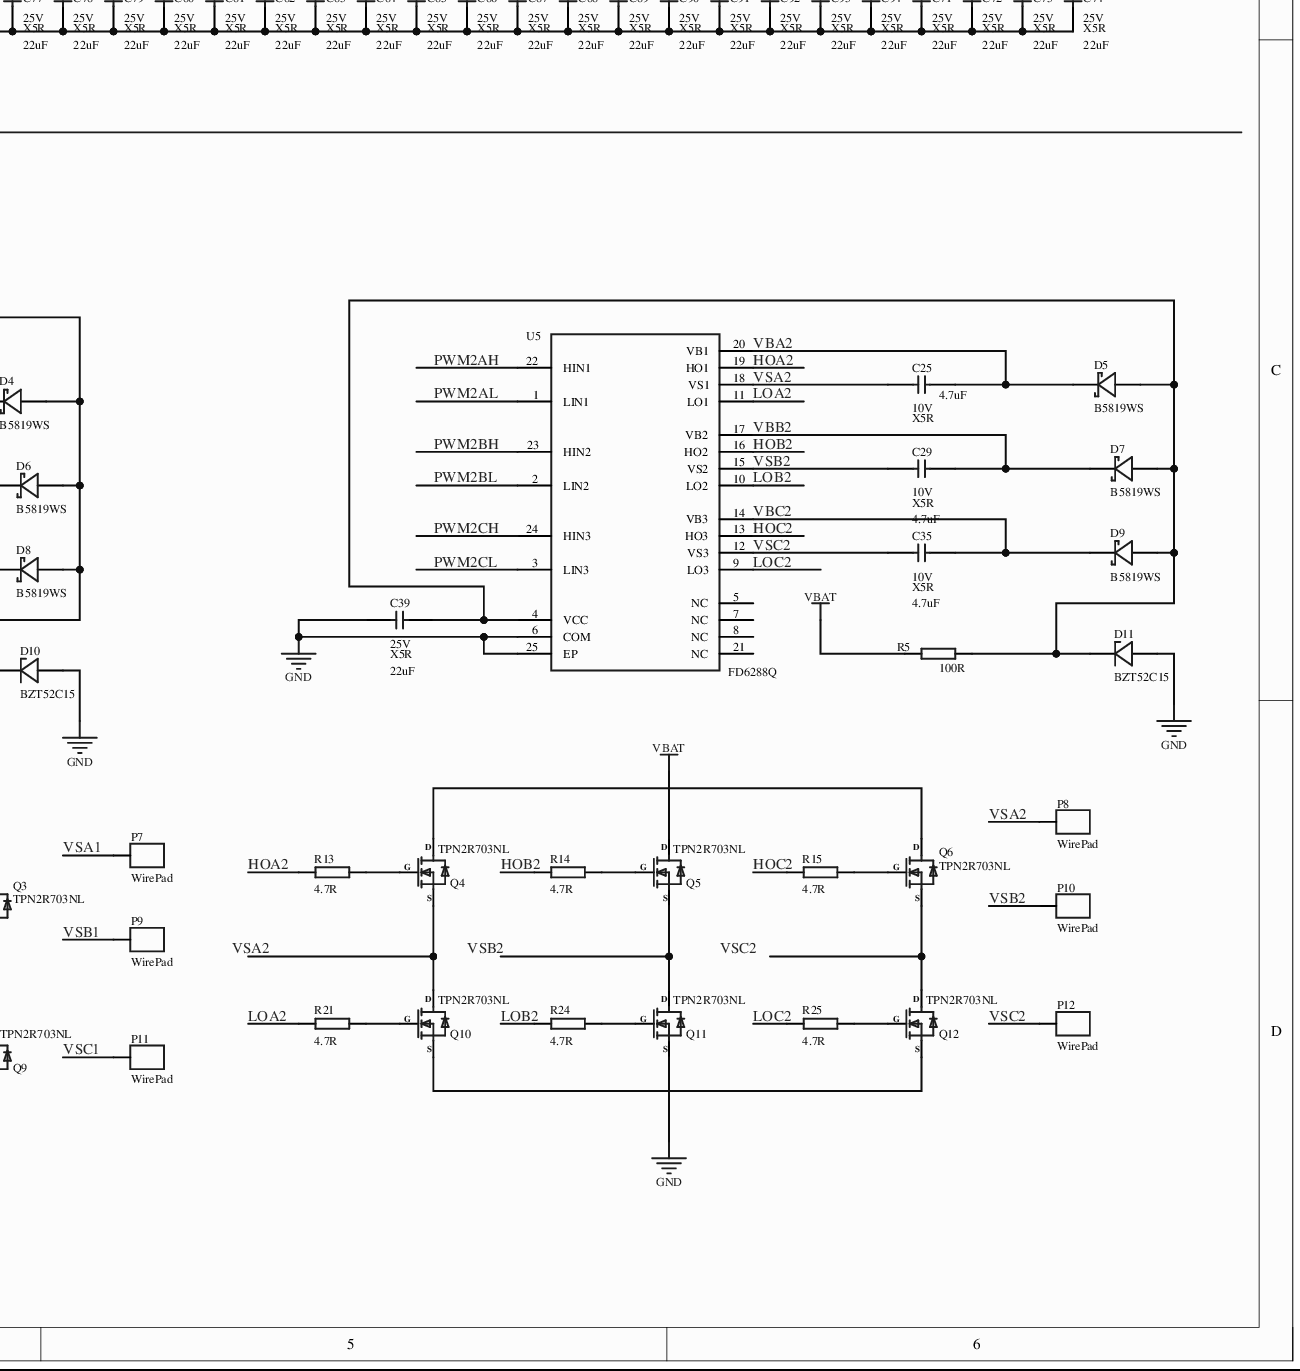
[diagram p0: MISC49862-3.schdoc, bottom right]
# Altium project MISC49862-2.PrjPcb (part 3 of 4)
## Sheet MISC49862-3.schdoc (continued)
### Library data of the parts (continued)
C71 = =Value +' '+ Voltage + ' ' + Type: SMD ceramic capacitor; MLCC; 0805(2012);; Device: 22uF 25V X5R; Symbol: 22uF 0805 25V X5R; Origin Footprint 2: CAPC2012[0805]; Origin Footprint 3: CAPC2012[0805]S-L; Origin Footprint 4: CAPC2012[0805]S-M; UniqueId: 13c458815c86755b; AddInBom: yes; Origin Footprint 1: CAPC2012[0805]S-N; Design Item ID: 22uF 0805 25V X5R; Library Name: SEEKFREE_Capacitor; Revision: V1.0; FootprintName: CAPC2012[0805]S-N; ConvertToPcb: yes
C72 = =Value +' '+ Voltage + ' ' + Type: SMD ceramic capacitor; MLCC; 0805(2012);; Device: 22uF 25V X5R; Symbol: 22uF 0805 25V X5R; Origin Footprint 2: CAPC2012[0805]; Origin Footprint 3: CAPC2012[0805]S-L; Origin Footprint 4: CAPC2012[0805]S-M; UniqueId: 4c445f6b18a98c19; AddInBom: yes; Origin Footprint 1: CAPC2012[0805]S-N; Design Item ID: 22uF 0805 25V X5R; Library Name: SEEKFREE_Capacitor; Revision: V1.0; FootprintName: CAPC2012[0805]S-N; ConvertToPcb: yes
C73 = =Value +' '+ Voltage + ' ' + Type: SMD ceramic capacitor; MLCC; 0805(2012);; Device: 22uF 25V X5R; Symbol: 22uF 0805 25V X5R; Origin Footprint 2: CAPC2012[0805]; Origin Footprint 3: CAPC2012[0805]S-L; Origin Footprint 4: CAPC2012[0805]S-M; UniqueId: ed67743022cf1596; AddInBom: yes; Origin Footprint 1: CAPC2012[0805]S-N; Design Item ID: 22uF 0805 25V X5R; Library Name: SEEKFREE_Capacitor; Revision: V1.0; FootprintName: CAPC2012[0805]S-N; ConvertToPcb: yes
C74 = =Value +' '+ Voltage + ' ' + Type: SMD ceramic capacitor; MLCC; 0805(2012);; Device: 22uF 25V X5R; Symbol: 22uF 0805 25V X5R; Origin Footprint 2: CAPC2012[0805]; Origin Footprint 3: CAPC2012[0805]S-L; Origin Footprint 4: CAPC2012[0805]S-M; UniqueId: 428606a84a8f4e02; AddInBom: yes; Origin Footprint 1: CAPC2012[0805]S-N; Design Item ID: 22uF 0805 25V X5R; Library Name: SEEKFREE_Capacitor; Revision: V1.0; FootprintName: CAPC2012[0805]S-N; ConvertToPcb: yes
C75 = =Value +' '+ Voltage + ' ' + Type: SMD ceramic capacitor; MLCC; 0805(2012);; Device: 22uF 25V X5R; Symbol: 22uF 0805 25V X5R; Origin Footprint 2: CAPC2012[0805]; Origin Footprint 3: CAPC2012[0805]S-L; Origin Footprint 4: CAPC2012[0805]S-M; UniqueId: 94802851accbed84; AddInBom: yes; Origin Footprint 1: CAPC2012[0805]S-N; Design Item ID: 22uF 0805 25V X5R; Library Name: SEEKFREE_Capacitor; Revision: V1.0; FootprintName: CAPC2012[0805]S-N; ConvertToPcb: yes
C76 = =Value +' '+ Voltage + ' ' + Type: SMD ceramic capacitor; MLCC; 0805(2012);; Device: 22uF 25V X5R; Symbol: 22uF 0805 25V X5R; Origin Footprint 2: CAPC2012[0805]; Origin Footprint 3: CAPC2012[0805]S-L; Origin Footprint 4: CAPC2012[0805]S-M; UniqueId: e46c4319d3798579; AddInBom: yes; Origin Footprint 1: CAPC2012[0805]S-N; Design Item ID: 22uF 0805 25V X5R; Library Name: SEEKFREE_Capacitor; Revision: V1.0; FootprintName: CAPC2012[0805]S-N; ConvertToPcb: yes
C77 = =Value +' '+ Voltage + ' ' + Type: SMD ceramic capacitor; MLCC; 0805(2012);; Device: 22uF 25V X5R; Symbol: 22uF 0805 25V X5R; Origin Footprint 2: CAPC2012[0805]; Origin Footprint 3: CAPC2012[0805]S-L; Origin Footprint 4: CAPC2012[0805]S-M; UniqueId: d85eccf1df583bf1; AddInBom: yes; Origin Footprint 1: CAPC2012[0805]S-N; Design Item ID: 22uF 0805 25V X5R; Library Name: SEEKFREE_Capacitor; Revision: V1.0; FootprintName: CAPC2012[0805]S-N; ConvertToPcb: yes
C78 = =Value +' '+ Voltage + ' ' + Type: SMD ceramic capacitor; MLCC; 0805(2012);; Device: 22uF 25V X5R; Symbol: 22uF 0805 25V X5R; Origin Footprint 2: CAPC2012[0805]; Origin Footprint 3: CAPC2012[0805]S-L; Origin Footprint 4: CAPC2012[0805]S-M; UniqueId: 289a7498a46a83c5; AddInBom: yes; Origin Footprint 1: CAPC2012[0805]S-N; Design Item ID: 22uF 0805 25V X5R; Library Name: SEEKFREE_Capacitor; Revision: V1.0; FootprintName: CAPC2012[0805]S-N; ConvertToPcb: yes
C79 = =Value +' '+ Voltage + ' ' + Type: SMD ceramic capacitor; MLCC; 0805(2012);; Device: 22uF 25V X5R; Symbol: 22uF 0805 25V X5R; Origin Footprint 2: CAPC2012[0805]; Origin Footprint 3: CAPC2012[0805]S-L; Origin Footprint 4: CAPC2012[0805]S-M; UniqueId: 1d1687b72a359977; AddInBom: yes; Origin Footprint 1: CAPC2012[0805]S-N; Design Item ID: 22uF 0805 25V X5R; Library Name: SEEKFREE_Capacitor; Revision: V1.0; FootprintName: CAPC2012[0805]S-N; ConvertToPcb: yes
C80 = =Value +' '+ Voltage + ' ' + Type: SMD ceramic capacitor; MLCC; 0805(2012);; Device: 22uF 25V X5R; Symbol: 22uF 0805 25V X5R; Origin Footprint 2: CAPC2012[0805]; Origin Footprint 3: CAPC2012[0805]S-L; Origin Footprint 4: CAPC2012[0805]S-M; UniqueId: 2dbd9816442fdb9a; AddInBom: yes; Origin Footprint 1: CAPC2012[0805]S-N; Design Item ID: 22uF 0805 25V X5R; Library Name: SEEKFREE_Capacitor; Revision: V1.0; FootprintName: CAPC2012[0805]S-N; ConvertToPcb: yes
C81 = =Value +' '+ Voltage + ' ' + Type: SMD ceramic capacitor; MLCC; 0805(2012);; Device: 22uF 25V X5R; Symbol: 22uF 0805 25V X5R; Origin Footprint 2: CAPC2012[0805]; Origin Footprint 3: CAPC2012[0805]S-L; Origin Footprint 4: CAPC2012[0805]S-M; UniqueId: bdf2686215596067; AddInBom: yes; Origin Footprint 1: CAPC2012[0805]S-N; Design Item ID: 22uF 0805 25V X5R; Library Name: SEEKFREE_Capacitor; Revision: V1.0; FootprintName: CAPC2012[0805]S-N; ConvertToPcb: yes
C82 = =Value +' '+ Voltage + ' ' + Type: SMD ceramic capacitor; MLCC; 0805(2012);; Device: 22uF 25V X5R; Symbol: 22uF 0805 25V X5R; Origin Footprint 2: CAPC2012[0805]; Origin Footprint 3: CAPC2012[0805]S-L; Origin Footprint 4: CAPC2012[0805]S-M; UniqueId: 2ac4a713bdb27458; AddInBom: yes; Origin Footprint 1: CAPC2012[0805]S-N; Design Item ID: 22uF 0805 25V X5R; Library Name: SEEKFREE_Capacitor; Revision: V1.0; FootprintName: CAPC2012[0805]S-N; ConvertToPcb: yes
C83 = =Value +' '+ Voltage + ' ' + Type: SMD ceramic capacitor; MLCC; 0805(2012);; Device: 22uF 25V X5R; Symbol: 22uF 0805 25V X5R; Origin Footprint 2: CAPC2012[0805]; Origin Footprint 3: CAPC2012[0805]S-L; Origin Footprint 4: CAPC2012[0805]S-M; UniqueId: 2b2365c2d0e3ae99; AddInBom: yes; Origin Footprint 1: CAPC2012[0805]S-N; Design Item ID: 22uF 0805 25V X5R; Library Name: SEEKFREE_Capacitor; Revision: V1.0; FootprintName: CAPC2012[0805]S-N; ConvertToPcb: yes
C84 = =Value +' '+ Voltage + ' ' + Type: SMD ceramic capacitor; MLCC; 0805(2012);; Device: 22uF 25V X5R; Symbol: 22uF 0805 25V X5R; Origin Footprint 2: CAPC2012[0805]; Origin Footprint 3: CAPC2012[0805]S-L; Origin Footprint 4: CAPC2012[0805]S-M; UniqueId: ac7cf9eb5671d2c3; AddInBom: yes; Origin Footprint 1: CAPC2012[0805]S-N; Design Item ID: 22uF 0805 25V X5R; Library Name: SEEKFREE_Capacitor; Revision: V1.0; FootprintName: CAPC2012[0805]S-N; ConvertToPcb: yes
C85 = =Value +' '+ Voltage + ' ' + Type: SMD ceramic capacitor; MLCC; 0805(2012);; Device: 22uF 25V X5R; Symbol: 22uF 0805 25V X5R; Origin Footprint 2: CAPC2012[0805]; Origin Footprint 3: CAPC2012[0805]S-L; Origin Footprint 4: CAPC2012[0805]S-M; UniqueId: 6158349470ed1956; AddInBom: yes; Origin Footprint 1: CAPC2012[0805]S-N; Design Item ID: 22uF 0805 25V X5R; Library Name: SEEKFREE_Capacitor; Revision: V1.0; FootprintName: CAPC2012[0805]S-N; ConvertToPcb: yes
C86 = =Value +' '+ Voltage + ' ' + Type: SMD ceramic capacitor; MLCC; 0805(2012);; Device: 22uF 25V X5R; Symbol: 22uF 0805 25V X5R; Origin Footprint 2: CAPC2012[0805]; Origin Footprint 3: CAPC2012[0805]S-L; Origin Footprint 4: CAPC2012[0805]S-M; UniqueId: 043006a40a259ae3; AddInBom: yes; Origin Footprint 1: CAPC2012[0805]S-N; Design Item ID: 22uF 0805 25V X5R; Library Name: SEEKFREE_Capacitor; Revision: V1.0; FootprintName: CAPC2012[0805]S-N; ConvertToPcb: yes
C87 = =Value +' '+ Voltage + ' ' + Type: SMD ceramic capacitor; MLCC; 0805(2012);; Device: 22uF 25V X5R; Symbol: 22uF 0805 25V X5R; Origin Footprint 2: CAPC2012[0805]; Origin Footprint 3: CAPC2012[0805]S-L; Origin Footprint 4: CAPC2012[0805]S-M; UniqueId: ed052c5890e059ff; AddInBom: yes; Origin Footprint 1: CAPC2012[0805]S-N; Design Item ID: 22uF 0805 25V X5R; Library Name: SEEKFREE_Capacitor; Revision: V1.0; FootprintName: CAPC2012[0805]S-N; ConvertToPcb: yes
C88 = =Value +' '+ Voltage + ' ' + Type: SMD ceramic capacitor; MLCC; 0805(2012);; Device: 22uF 25V X5R; Symbol: 22uF 0805 25V X5R; Origin Footprint 2: CAPC2012[0805]; Origin Footprint 3: CAPC2012[0805]S-L; Origin Footprint 4: CAPC2012[0805]S-M; UniqueId: 909660952e1a96fd; AddInBom: yes; Origin Footprint 1: CAPC2012[0805]S-N; Design Item ID: 22uF 0805 25V X5R; Library Name: SEEKFREE_Capacitor; Revision: V1.0; FootprintName: CAPC2012[0805]S-N; ConvertToPcb: yes
C89 = =Value +' '+ Voltage + ' ' + Type: SMD ceramic capacitor; MLCC; 0805(2012);; Device: 22uF 25V X5R; Symbol: 22uF 0805 25V X5R; Origin Footprint 2: CAPC2012[0805]; Origin Footprint 3: CAPC2012[0805]S-L; Origin Footprint 4: CAPC2012[0805]S-M; UniqueId: f9bfd7a6531d354d; AddInBom: yes; Origin Footprint 1: CAPC2012[0805]S-N; Design Item ID: 22uF 0805 25V X5R; Library Name: SEEKFREE_Capacitor; Revision: V1.0; FootprintName: CAPC2012[0805]S-N; ConvertToPcb: yes
C90 = =Value +' '+ Voltage + ' ' + Type: SMD ceramic capacitor; MLCC; 0805(2012);; Device: 22uF 25V X5R; Symbol: 22uF 0805 25V X5R; Origin Footprint 2: CAPC2012[0805]; Origin Footprint 3: CAPC2012[0805]S-L; Origin Footprint 4: CAPC2012[0805]S-M; UniqueId: 5471cb5e6ead650e; AddInBom: yes; Origin Footprint 1: CAPC2012[0805]S-N; Design Item ID: 22uF 0805 25V X5R; Library Name: SEEKFREE_Capacitor; Revision: V1.0; FootprintName: CAPC2012[0805]S-N; ConvertToPcb: yes
C91 = =Value +' '+ Voltage + ' ' + Type: SMD ceramic capacitor; MLCC; 0805(2012);; Device: 22uF 25V X5R; Symbol: 22uF 0805 25V X5R; Origin Footprint 2: CAPC2012[0805]; Origin Footprint 3: CAPC2012[0805]S-L; Origin Footprint 4: CAPC2012[0805]S-M; UniqueId: de488198406d19e5; AddInBom: yes; Origin Footprint 1: CAPC2012[0805]S-N; Design Item ID: 22uF 0805 25V X5R; Library Name: SEEKFREE_Capacitor; Revision: V1.0; FootprintName: CAPC2012[0805]S-N; ConvertToPcb: yes
C92 = =Value +' '+ Voltage + ' ' + Type: SMD ceramic capacitor; MLCC; 0805(2012);; Device: 22uF 25V X5R; Symbol: 22uF 0805 25V X5R; Origin Footprint 2: CAPC2012[0805]; Origin Footprint 3: CAPC2012[0805]S-L; Origin Footprint 4: CAPC2012[0805]S-M; UniqueId: 7abe426619a81940; AddInBom: yes; Origin Footprint 1: CAPC2012[0805]S-N; Design Item ID: 22uF 0805 25V X5R; Library Name: SEEKFREE_Capacitor; Revision: V1.0; FootprintName: CAPC2012[0805]S-N; ConvertToPcb: yes
C93 = =Value +' '+ Voltage + ' ' + Type: SMD ceramic capacitor; MLCC; 0805(2012);; Device: 22uF 25V X5R; Symbol: 22uF 0805 25V X5R; Origin Footprint 2: CAPC2012[0805]; Origin Footprint 3: CAPC2012[0805]S-L; Origin Footprint 4: CAPC2012[0805]S-M; UniqueId: ecf0d2211b923647; AddInBom: yes; Origin Footprint 1: CAPC2012[0805]S-N; Design Item ID: 22uF 0805 25V X5R; Library Name: SEEKFREE_Capacitor; Revision: V1.0; FootprintName: CAPC2012[0805]S-N; ConvertToPcb: yes
C94 = =Value +' '+ Voltage + ' ' + Type: SMD ceramic capacitor; MLCC; 0805(2012);; Device: 22uF 25V X5R; Symbol: 22uF 0805 25V X5R; Origin Footprint 2: CAPC2012[0805]; Origin Footprint 3: CAPC2012[0805]S-L; Origin Footprint 4: CAPC2012[0805]S-M; UniqueId: 7c9a59bbe2a187d0; AddInBom: yes; Origin Footprint 1: CAPC2012[0805]S-N; Design Item ID: 22uF 0805 25V X5R; Library Name: SEEKFREE_Capacitor; Revision: V1.0; FootprintName: CAPC2012[0805]S-N; ConvertToPcb: yes
D1 = B5819WS: B5819WS Schottky diode; UniqueId: 6eb2f7ba7a12821c; AddInBom: yes; Origin Footprint: SOD-323; Device: B5819WS; Symbol: B5819WS; Design Item ID: B5819WS; Library Name: Brushless driver-CYT2BL3-FD6288-FOC-LiteDual; Revision: V1.0; Value: B5819WS; FootprintName: SOD-323; ConvertToPcb: yes
D3 = SMAJ16CA: TRANSIENT VOLTAGE  SUPPRESSOR DIODE; Symbol: Diode TVS Bi-Dir; Imax: 500mA; Origin Footprint 2: DO-41; Origin Footprint 3: SMA[DO-214AC]; Origin Footprint 4: SMB[DO-214AA]; Origin Footprint 5: SMC[DO-214AB]; Origin Footprint 6: SOD-123-FL; Origin Footprint 7: SOD-323; Origin Footprint 8: SOD-523-M; Origin Footprint 9: SOD-123-L; Origin Footprint 10: SOD-123-M; Origin Footprint 11: SOD-523-L; Origin Footprint 12: SMC[DO-214AB]-Bi; UniqueId: 81689f1d3303caec; AddInBom: yes; Origin Footprint 1: SMA[DO-214AC]-Bi; Device: SMAJ16CA; Design Item ID: Diode TVS Bi-Dir; Library Name: SEEKFREE_Diode; Published: 8-Jun-2000; Price(RMB): 0.000; FootprintName: SMA[DO-214AC]-Bi; ConvertToPcb: yes; Publisher: Altium Limited
D4 = B5819WS: B5819WS Schottky diode; UniqueId: 6a4368da87585c93; AddInBom: yes; Origin Footprint: SOD-323; Device: B5819WS; Symbol: B5819WS; Design Item ID: B5819WS; Library Name: SEEKFREE_Diode; Revision: V1.0; Value: B5819WS; FootprintName: SOD-323; ConvertToPcb: yes
D5 = B5819WS: B5819WS Schottky diode; UniqueId: aa27cf4c2f614704; AddInBom: yes; Origin Footprint: SOD-323; Device: B5819WS; Symbol: B5819WS; Design Item ID: B5819WS; Library Name: SEEKFREE_Diode; Revision: V1.0; Value: B5819WS; FootprintName: SOD-323; ConvertToPcb: yes
D6 = B5819WS: B5819WS Schottky diode; UniqueId: 0b466d7a0d9696a1; AddInBom: yes; Origin Footprint: SOD-323; Device: B5819WS; Symbol: B5819WS; Design Item ID: B5819WS; Library Name: SEEKFREE_Diode; Revision: V1.0; Value: B5819WS; FootprintName: SOD-323; ConvertToPcb: yes
D7 = B5819WS: B5819WS Schottky diode; UniqueId: 61ba849a9213f6b6; AddInBom: yes; Origin Footprint: SOD-323; Device: B5819WS; Symbol: B5819WS; Design Item ID: B5819WS; Library Name: SEEKFREE_Diode; Revision: V1.0; Value: B5819WS; FootprintName: SOD-323; ConvertToPcb: yes
D8 = B5819WS: B5819WS Schottky diode; UniqueId: d726a396729c3148; AddInBom: yes; Origin Footprint: SOD-323; Device: B5819WS; Symbol: B5819WS; Design Item ID: B5819WS; Library Name: SEEKFREE_Diode; Revision: V1.0; Value: B5819WS; FootprintName: SOD-323; ConvertToPcb: yes
D9 = B5819WS: B5819WS Schottky diode; UniqueId: ff0c81595de38f51; AddInBom: yes; Origin Footprint: SOD-323; Device: B5819WS; Symbol: B5819WS; Design Item ID: B5819WS; Library Name: SEEKFREE_Diode; Revision: V1.0; Value: B5819WS; FootprintName: SOD-323; ConvertToPcb: yes
D10 = BZT52C15: Zener diode (voltage regulator); Symbol: Diode Zen; Origin Footprint 2: DIODE-0.7; Origin Footprint 3: DIODE-0.4; Origin Footprint 4: SOD-87[LL-41]; Origin Footprint 5: CD4521-1808; Origin Footprint 6: SOD-80[LL-34]; Origin Footprint 7: SOD-123-FL; Origin Footprint 8: SOD-123-M; Origin Footprint 9: SOD-323; Origin Footprint 10: SOD-523-L; Origin Footprint 11: SOD-523-M; UniqueId: 260e63abbc5bbcdd; AddInBom: yes; Origin Footprint 1: SOD-123-L; Device: BZT52C15; Design Item ID: Diode Zen; Library Name: SEEKFREE_Diode; Published: 8-Jun-2000; Revision: July-2002: Re-released for DXP Platform.; Price(RMB): 0.000; FootprintName: SOD-123-L; ConvertToPcb: yes; Publisher: Altium Limited
D11 = BZT52C15: Zener diode (voltage regulator); Symbol: Diode Zen; Origin Footprint 2: DIODE-0.7; Origin Footprint 3: DIODE-0.4; Origin Footprint 4: SOD-87[LL-41]; Origin Footprint 5: CD4521-1808; Origin Footprint 6: SOD-80[LL-34]; Origin Footprint 7: SOD-123-FL; Origin Footprint 8: SOD-123-M; Origin Footprint 9: SOD-323; Origin Footprint 10: SOD-523-L; Origin Footprint 11: SOD-523-M; UniqueId: 63002c75ba05748a; AddInBom: yes; Origin Footprint 1: SOD-123-L; Device: BZT52C15; Design Item ID: Diode Zen; Library Name: SEEKFREE_Diode; Published: 8-Jun-2000; Revision: July-2002: Re-released for DXP Platform.; Price(RMB): 0.000; FootprintName: SOD-123-L; ConvertToPcb: yes; Publisher: Altium Limited
D12 = SMF3.3A: TRANSIENT VOLTAGE  SUPPRESSOR DIODE; Symbol: Diode TVS Uni-Dir; Imax: 500mA; Origin Footprint 2: DO-41; Origin Footprint 3: SMA[DO-214AC]; Origin Footprint 4: SMB[DO-214AA]; Origin Footprint 5: SMC[DO-214AB]; Origin Footprint 6: SOD-323; Origin Footprint 7: SOD-123-L; Origin Footprint 8: SOD-523-L; Origin Footprint 9: SOD-123-M; Origin Footprint 10: SOD-523-M; UniqueId: a80f7d1f54f711b8; AddInBom: yes; Origin Footprint 1: SOD-123-FL; Device: SMF3.3A; Design Item ID: Diode TVS Uni-Dir; Library Name: Brushless driver-CYT2BL3-FD6288-FOC-LiteDual; Published: 8-Jun-2000; Price(RMB): 0.000; FootprintName: SOD-123-FL; ConvertToPcb: yes; Publisher: Altium Limited
D13 = B5819WS: B5819WS Schottky diode; UniqueId: d3460379f3d05a2a; AddInBom: yes; Origin Footprint: SOD-323; Device: B5819WS; Symbol: B5819WS; Design Item ID: B5819WS; Library Name: Brushless driver-CYT2BL3-FD6288-FOC-LiteDual; Revision: V1.0; Value: B5819WS; FootprintName: SOD-323; ConvertToPcb: yes
D14 = SMAJ16CA: TRANSIENT VOLTAGE  SUPPRESSOR DIODE; Symbol: Diode TVS Bi-Dir; Imax: 500mA; Origin Footprint 2: DO-41; Origin Footprint 3: SMA[DO-214AC]; Origin Footprint 4: SMB[DO-214AA]; Origin Footprint 5: SMC[DO-214AB]; Origin Footprint 6: SOD-123-FL; Origin Footprint 7: SOD-323; Origin Footprint 8: SOD-523-M; Origin Footprint 9: SOD-123-L; Origin Footprint 10: SOD-123-M; Origin Footprint 11: SOD-523-L; Origin Footprint 12: SMC[DO-214AB]-Bi; UniqueId: f1c346e37d3cba37; AddInBom: yes; Origin Footprint 1: SMA[DO-214AC]-Bi; Device: SMAJ16CA; Design Item ID: Diode TVS Bi-Dir; Library Name: SEEKFREE_Diode; Published: 8-Jun-2000; Price(RMB): 0.000; FootprintName: SMA[DO-214AC]-Bi; ConvertToPcb: yes; Publisher: Altium Limited
FB1 = =Value + ' ' + Frequency +' '+ Imax: SMD ferrite bead; Device: 120R @100MHz 500mA; Symbol: FB-Chip; DCR: .1m; Frequency: @100MHz; Imax: 500mA; Origin Footprint 2: INDC1608[0603]S; Origin Footprint 3: INDC2012[0805]S; Origin Footprint 4: INDC3216[1206]S; Origin Footprint 5: INDC4509[1806]S; Origin Footprint 6: INDC1005[0402]; Origin Footprint 7: INDC1608[0603]; Origin Footprint 8: INDC2012[0805]; Origin Footprint 9: INDC3216[1206]; Origin Footprint 10: INDC3225[1210]; UniqueId: 323bb55b4674cf0d; AddInBom: yes; Origin Footprint 1: INDC1005[0402]S; Design Item ID: FB-Chip; Library Name: Brushless driver-CYT2BL3-FD6288-FOC-LiteDual; Published: 2020-12-18; Revision: V1.0; Origin Footprint 11: INDC3216[1206]; FootprintName: INDC1005[0402]S; ConvertToPcb: yes
FB2 = =Value + ' ' + Frequency +' '+ Imax: SMD ferrite bead; Device: 120R @100MHz 500mA; Symbol: FB-Chip; DCR: .1m; Frequency: @100MHz; Imax: 500mA; Origin Footprint 2: INDC1608[0603]S; Origin Footprint 3: INDC2012[0805]S; Origin Footprint 4: INDC3216[1206]S; Origin Footprint 5: INDC4509[1806]S; Origin Footprint 6: INDC1005[0402]; Origin Footprint 7: INDC1608[0603]; Origin Footprint 8: INDC2012[0805]; Origin Footprint 9: INDC3216[1206]; Origin Footprint 10: INDC3225[1210]; UniqueId: 62384c8cdaa0e7c8; AddInBom: yes; Origin Footprint 1: INDC1005[0402]S; Design Item ID: FB-Chip; Library Name: Brushless driver-CYT2BL3-FD6288-FOC-LiteDual; Published: 2020-12-18; Revision: V1.0; Origin Footprint 11: INDC3216[1206]; FootprintName: INDC1005[0402]S; ConvertToPcb: yes
L1 = =Value + ' ' + Imax: Power inductor; Device: 4.7uH 2A; Symbol: Ind-Power; DCR: .5m; Origin Footprint 2: CD31; Origin Footprint 3: CD32; Origin Footprint 4: CD42; Origin Footprint 5: CD43; Origin Footprint 6: CD52; Origin Footprint 7: CD53; Origin Footprint 8: CD54; Origin Footprint 9: CD73; Origin Footprint 10: CD75; Origin Footprint 11: CD104; Origin Footprint 12: CD105; Origin Footprint 13: CD106; Origin Footprint 14: 127 Shielded 12.5*12.5*7; Origin Footprint 15: 0630 TPC 7*7*3; Origin Footprint 16: 1050 TPC 10*10*5; Origin Footprint 17: 1265 TPC 12*12*6.5; Origin Footprint 18: CD104R; Origin Footprint 19: 1365 TPC 13*13*6.5; Origin Footprint 21: 0402 TPC 4*4*2; UniqueId: d450ceac7adb81c3; AddInBom: yes; Origin Footprint 1: SLO2520; Design Item ID: Ind-Power; Library Name: Brushless driver-CYT2BL3-FD6288-FOC-LiteDual; Published: 8-Jun-2000; Revision: July-2002: Re-released for DXP Platform.; Price(RMB): 0.000; Origin Footprint 20: INDUCTOR; FootprintName: SLO2520; ConvertToPcb: yes; Publisher: Altium Limited
L2 = =Value + ' ' + Imax: Power inductor; Device: 4.7uH 2A; Symbol: Ind-Power; DCR: .5m; Origin Footprint 2: CD31; Origin Footprint 3: CD32; Origin Footprint 4: CD42; Origin Footprint 5: CD43; Origin Footprint 6: CD52; Origin Footprint 7: CD53; Origin Footprint 8: CD54; Origin Footprint 9: CD73; Origin Footprint 10: CD75; Origin Footprint 11: CD104; Origin Footprint 12: CD105; Origin Footprint 13: CD106; Origin Footprint 14: 127 Shielded 12.5*12.5*7; Origin Footprint 15: 0630 TPC 7*7*3; Origin Footprint 16: 1050 TPC 10*10*5; Origin Footprint 17: 1265 TPC 12*12*6.5; Origin Footprint 18: CD104R; Origin Footprint 19: 1365 TPC 13*13*6.5; Origin Footprint 21: 0402 TPC 4*4*2; UniqueId: 3f6ee2b1a34b017f; AddInBom: yes; Origin Footprint 1: SLO2520; Design Item ID: Ind-Power; Library Name: Brushless driver-CYT2BL3-FD6288-FOC-LiteDual; Published: 8-Jun-2000; Revision: July-2002: Re-released for DXP Platform.; Price(RMB): 0.000; Origin Footprint 20: INDUCTOR; FootprintName: SLO2520; ConvertToPcb: yes; Publisher: Altium Limited
LED1 = 红色贴片LED: Symbol: LED Chip Red; Origin Footprint 2: LEDC1608(0603); Origin Footprint 3: LEDC2012(0805); Origin Footprint 4: LEDC3216(1206); Origin Footprint 5: LEDC2012(0805)-L; Origin Footprint 6: LEDC3216(1204); Origin Footprint 7: LEDC3528-2; UniqueId: 7a65b453ee5a9ec2; AddInBom: yes; Origin Footprint 1: LEDC1608(0603)-L; Device: Red SMD LED; Design Item ID: LED Chip Red; Library Name: Brushless driver-CYT2BL3-FD6288-FOC-LiteDual; Published: 8-Jun-2000; Revision: July-2002: Re-released for DXP Platform.; Price(RMB): 0.00; Description: Red SMD LED; FootprintName: LEDC1608(0603)-L; ConvertToPcb: yes; Publisher: Altium Limited
LED2 = 蓝色贴片LED: Symbol: LED Chip Blue; Origin Footprint 2: LEDC1608(0603); Origin Footprint 3: LEDC2012(0805); Origin Footprint 4: LEDC3216(1206); Origin Footprint 5: LEDC2012(0805)-L; Origin Footprint 6: LEDC3216(1204); Origin Footprint 7: LEDC3528-2; UniqueId: 48c2d4982f4ec99a; AddInBom: yes; Origin Footprint 1: LEDC1608(0603)-L; Device: Blue SMD LED; Design Item ID: LED Chip Blue; Library Name: Brushless driver-CYT2BL3-FD6288-FOC-LiteDual; Published: 8-Jun-2000; Revision: July-2002: Re-released for DXP Platform.; Price(RMB): 0.00; Color: Blue; Description: Blue SMD LED; FootprintName: LEDC1608(0603)-L; ConvertToPcb: yes; Publisher: Altium Limited
P1 = SWD Header 5x2: SWD debug interface 2x5pin dual-row pin header; Origin Footprint 2: HDR2X5-M-SMT; Origin Footprint 3: HDR2X5-M; Origin Footprint 4: IDC2.54-10-DV; Origin Footprint 5: IDC2.54-10-SV; Origin Footprint 6: IDC2.54-10-DH; UniqueId: c39ee3c861a7b382; AddInBom: yes; Origin Footprint 1: HDR2X5-OB; Device: SWD Header 5x2; Symbol: SWD Header 5x2; Design Item ID: SWD Header 5x2; Library Name: Brushless driver-CYT2BL3-FD6288-FOC-LiteDual; Revision: V1.0; FootprintName: HDR2X5-OB; ConvertToPcb: yes
P2 = XH2.54-3P: Origin Footprint 2: XH2.54-3P-DH; Origin Footprint 3: XH2.54-3P-DV; UniqueId: 16cbebb8866e1842; AddInBom: yes; Origin Footprint 1: XH2.54-3P-SH; Device: XH2.54-3P; Symbol: XH2.54-3P; Design Item ID: XH2.54-3P; Library Name: Brushless driver-CYT2BL3-FD6288-FOC-LiteDual; Revision: V1.0; Value: XH2.54-3P; Description: XH2.54-3P; FootprintName: XH2.54-3P-SH; ConvertToPcb: yes
P3 = ZH1.5-6P: Origin Footprint 2: ZH1.5-6P-DV; UniqueId: 1bc31e334497ec54; AddInBom: yes; Origin Footprint 1: ZH1.5-6P-SH; Device: ZH1.5-6P; Symbol: ZH1.5-6P; Design Item ID: ZH1.5-6P; Library Name: Brushless driver-CYT2BL3-FD6288-FOC-LiteDual; Revision: V1.0; Value: ZH1.5-6P; Description: ZH1.5-6P; FootprintName: ZH1.5-6P-SH; ConvertToPcb: yes
P4 = ZH1.5-6P: Origin Footprint 2: ZH1.5-6P-DV; UniqueId: 6a809a8f8408ed49; AddInBom: yes; Origin Footprint 1: ZH1.5-6P-SH; Device: ZH1.5-6P; Symbol: ZH1.5-6P; Design Item ID: ZH1.5-6P; Library Name: Brushless driver-CYT2BL3-FD6288-FOC-LiteDual; Revision: V1.0; Value: ZH1.5-6P; Description: ZH1.5-6P; FootprintName: ZH1.5-6P-SH; ConvertToPcb: yes
P5 = WirePad: Cable wire pad; Origin Footprint 2: WirePad-4.5x7; UniqueId: a30bd92ff87464e3; AddInBom: yes; Origin Footprint 1: WirePad-4x6; Device: WirePad; Symbol: WirePad; Design Item ID: WirePad; Library Name: SEEKFREE_Connector; FootprintName: WirePad-4x6; ConvertToPcb: yes
P6 = WirePad: Cable wire pad; Origin Footprint 2: WirePad-4.5x7; UniqueId: 2d4d75c2fcc000cd; AddInBom: yes; Origin Footprint 1: WirePad-4x6; Device: WirePad; Symbol: WirePad; Design Item ID: WirePad; Library Name: SEEKFREE_Connector; FootprintName: WirePad-4x6; ConvertToPcb: yes
P7 = WirePad: Cable wire pad; Origin Footprint 2: WirePad-4.5x7; UniqueId: f2444bf4b29cd8fb; AddInBom: yes; Origin Footprint 1: WirePad-4x6; Device: WirePad; Symbol: WirePad; Design Item ID: WirePad; Library Name: SEEKFREE_Connector; FootprintName: WirePad-4x6; ConvertToPcb: yes
P8 = WirePad: Cable wire pad; Origin Footprint 2: WirePad-4.5x7; UniqueId: c12bb200b862f639; AddInBom: yes; Origin Footprint 1: WirePad-4x6; Device: WirePad; Symbol: WirePad; Design Item ID: WirePad; Library Name: SEEKFREE_Connector; FootprintName: WirePad-4x6; ConvertToPcb: yes
P9 = WirePad: Cable wire pad; Origin Footprint 2: WirePad-4.5x7; UniqueId: 0372b66f43e88ef3; AddInBom: yes; Origin Footprint 1: WirePad-4x6; Device: WirePad; Symbol: WirePad; Design Item ID: WirePad; Library Name: SEEKFREE_Connector; FootprintName: WirePad-4x6; ConvertToPcb: yes
P10 = WirePad: Cable wire pad; Origin Footprint 2: WirePad-4.5x7; UniqueId: 5e10277718398939; AddInBom: yes; Origin Footprint 1: WirePad-4x6; Device: WirePad; Symbol: WirePad; Design Item ID: WirePad; Library Name: SEEKFREE_Connector; FootprintName: WirePad-4x6; ConvertToPcb: yes
P11 = WirePad: Cable wire pad; Origin Footprint 2: WirePad-4.5x7; UniqueId: e3530c10d10e903a; AddInBom: yes; Origin Footprint 1: WirePad-4x6; Device: WirePad; Symbol: WirePad; Design Item ID: WirePad; Library Name: SEEKFREE_Connector; FootprintName: WirePad-4x6; ConvertToPcb: yes
P12 = WirePad: Cable wire pad; Origin Footprint 2: WirePad-4.5x7; UniqueId: 0618e235635c86ae; AddInBom: yes; Origin Footprint 1: WirePad-4x6; Device: WirePad; Symbol: WirePad; Design Item ID: WirePad; Library Name: SEEKFREE_Connector; FootprintName: WirePad-4x6; ConvertToPcb: yes
Q1 = TPN2R703NL: Toshiba N-channel MOS; UniqueId: f76c01de5337d462; AddInBom: yes; Origin Footprint: TSON3x3; Device: TPN2R703NL; Symbol: TPN2R703NL; Design Item ID: TPN2R703NL; Library Name: SEEKFREE_MOSFET; FootprintName: TSON3x3; ConvertToPcb: yes
Q2 = TPN2R703NL: Toshiba N-channel MOS; UniqueId: 4c27cd76e8dbac26; AddInBom: yes; Origin Footprint: TSON3x3; Device: TPN2R703NL; Symbol: TPN2R703NL; Design Item ID: TPN2R703NL; Library Name: SEEKFREE_MOSFET; FootprintName: TSON3x3; ConvertToPcb: yes
Q3 = TPN2R703NL: Toshiba N-channel MOS; UniqueId: 200f6e823ef85d95; AddInBom: yes; Origin Footprint: TSON3x3; Device: TPN2R703NL; Symbol: TPN2R703NL; Design Item ID: TPN2R703NL; Library Name: SEEKFREE_MOSFET; FootprintName: TSON3x3; ConvertToPcb: yes
Q4 = TPN2R703NL: Toshiba N-channel MOS; UniqueId: 2147c8f490bf262b; AddInBom: yes; Origin Footprint: TSON3x3; Device: TPN2R703NL; Symbol: TPN2R703NL; Design Item ID: TPN2R703NL; Library Name: SEEKFREE_MOSFET; FootprintName: TSON3x3; ConvertToPcb: yes
Q5 = TPN2R703NL: Toshiba N-channel MOS; UniqueId: c2db9f210f8adeb4; AddInBom: yes; Origin Footprint: TSON3x3; Device: TPN2R703NL; Symbol: TPN2R703NL; Design Item ID: TPN2R703NL; Library Name: SEEKFREE_MOSFET; FootprintName: TSON3x3; ConvertToPcb: yes
Q6 = TPN2R703NL: Toshiba N-channel MOS; UniqueId: a2a88fc5b0e77289; AddInBom: yes; Origin Footprint: TSON3x3; Device: TPN2R703NL; Symbol: TPN2R703NL; Design Item ID: TPN2R703NL; Library Name: SEEKFREE_MOSFET; FootprintName: TSON3x3; ConvertToPcb: yes
Q7 = TPN2R703NL: Toshiba N-channel MOS; UniqueId: 82fefbdc6423ee95; AddInBom: yes; Origin Footprint: TSON3x3; Device: TPN2R703NL; Symbol: TPN2R703NL; Design Item ID: TPN2R703NL; Library Name: SEEKFREE_MOSFET; FootprintName: TSON3x3; ConvertToPcb: yes
Q8 = TPN2R703NL: Toshiba N-channel MOS; UniqueId: 2ed88cf594e53a98; AddInBom: yes; Origin Footprint: TSON3x3; Device: TPN2R703NL; Symbol: TPN2R703NL; Design Item ID: TPN2R703NL; Library Name: SEEKFREE_MOSFET; FootprintName: TSON3x3; ConvertToPcb: yes
Q9 = TPN2R703NL: Toshiba N-channel MOS; UniqueId: 9a636d96af8c71e3; AddInBom: yes; Origin Footprint: TSON3x3; Device: TPN2R703NL; Symbol: TPN2R703NL; Design Item ID: TPN2R703NL; Library Name: SEEKFREE_MOSFET; FootprintName: TSON3x3; ConvertToPcb: yes
Q10 = TPN2R703NL: Toshiba N-channel MOS; UniqueId: c38283ed4a9e40e7; AddInBom: yes; Origin Footprint: TSON3x3; Device: TPN2R703NL; Symbol: TPN2R703NL; Design Item ID: TPN2R703NL; Library Name: SEEKFREE_MOSFET; FootprintName: TSON3x3; ConvertToPcb: yes
Q11 = TPN2R703NL: Toshiba N-channel MOS; UniqueId: e07807db00124b08; AddInBom: yes; Origin Footprint: TSON3x3; Device: TPN2R703NL; Symbol: TPN2R703NL; Design Item ID: TPN2R703NL; Library Name: SEEKFREE_MOSFET; FootprintName: TSON3x3; ConvertToPcb: yes
Q12 = TPN2R703NL: Toshiba N-channel MOS; UniqueId: 8276e929479111f4; AddInBom: yes; Origin Footprint: TSON3x3; Device: TPN2R703NL; Symbol: TPN2R703NL; Design Item ID: TPN2R703NL; Library Name: SEEKFREE_MOSFET; FootprintName: TSON3x3; ConvertToPcb: yes
R1 = =Value+' '+Tolerance: SMD resistor; Device: 10K ±1%; Symbol: Res-Chip_1; Tolerance: ±1%; Origin Footprint 2: RESC0603[0201]-L; Origin Footprint 3: RESC0603[0201]-M; Origin Footprint 4: RESC0603[0201]-N; Origin Footprint 5: RESC0603[0201]S-L; Origin Footprint 6: RESC0603[0201]S-M; Origin Footprint 7: RESC0603[0201]S-N; Origin Footprint 8: RESC1005[0402]-L; Origin Footprint 9: RESC1005[0402]-M; Origin Footprint 10: RESC1005[0402]-N; Origin Footprint 11: RESC1005[0402]S-L; Origin Footprint 12: RESC1005[0402]S-M; Origin Footprint 13: RESC1608[0603]-L; Origin Footprint 14: RESC1608[0603]-M; Origin Footprint 15: RESC1608[0603]-N; Origin Footprint 16: RESC1608[0603]S-L; Origin Footprint 17: RESC1608[0603]S-M; Origin Footprint 18: RESC1608[0603]S-N; Origin Footprint 19: RESC2012[0805]; Origin Footprint 20: RESC2012[0805]S-L; Origin Footprint 21: RESC2012[0805]S-M; Origin Footprint 22: RESC2012[0805]S-N; Origin Footprint 23: RESC3216[1206]; Origin Footprint 24: RESC3216[1206]S-L; Origin Footprint 25: RESC3216[1206]S-M; Origin Footprint 26: RESC3216[1206]S-N; Origin Footprint 27: RESC3225[1210]; Origin Footprint 28: RESC3225[1210]S; Origin Footprint 29: RESC5025[2010]; Origin Footprint 30: RESC5025[2010]S; Origin Footprint 31: RESC6332[2512]; Origin Footprint 32: RESC6332[2512]S; UniqueId: 353b166cc2dee846; AddInBom: yes; Origin Footprint 1: RESC1005[0402]S-N; Design Item ID: Res-Chip_1; Library Name: Brushless driver-CYT2BL3-FD6288-FOC-LiteDual; Revision: V1.0; FootprintName: RESC1005[0402]S-N; ConvertToPcb: yes
R2 = =Value+' '+Tolerance: SMD resistor; Device: 0R ±1%; Symbol: Res-Chip_2; Tolerance: ±1%; Origin Footprint 2: RESC0603[0201]-L; Origin Footprint 3: RESC0603[0201]-M; Origin Footprint 4: RESC0603[0201]-N; Origin Footprint 5: RESC0603[0201]S-L; Origin Footprint 6: RESC0603[0201]S-M; Origin Footprint 7: RESC0603[0201]S-N; Origin Footprint 8: RESC1005[0402]-L; Origin Footprint 9: RESC1005[0402]-M; Origin Footprint 10: RESC1005[0402]-N; Origin Footprint 11: RESC1005[0402]S-L; Origin Footprint 12: RESC1005[0402]S-M; Origin Footprint 13: RESC1608[0603]-L; Origin Footprint 14: RESC1608[0603]-M; Origin Footprint 15: RESC1608[0603]-N; Origin Footprint 16: RESC1608[0603]S-L; Origin Footprint 17: RESC1608[0603]S-M; Origin Footprint 18: RESC1608[0603]S-N; Origin Footprint 19: RESC2012[0805]; Origin Footprint 20: RESC2012[0805]S-L; Origin Footprint 21: RESC2012[0805]S-M; Origin Footprint 22: RESC2012[0805]S-N; Origin Footprint 23: RESC3216[1206]; Origin Footprint 24: RESC3216[1206]S-L; Origin Footprint 25: RESC3216[1206]S-M; Origin Footprint 26: RESC3216[1206]S-N; Origin Footprint 27: RESC3225[1210]; Origin Footprint 28: RESC3225[1210]S; Origin Footprint 29: RESC5025[2010]; Origin Footprint 30: RESC5025[2010]S; Origin Footprint 31: RESC6332[2512]; Origin Footprint 32: RESC6332[2512]S; UniqueId: 6f63fc6711cfa315; AddInBom: yes; Origin Footprint 1: RESC1005[0402]S-N; Design Item ID: Res-Chip_2; Library Name: Brushless driver-CYT2BL3-FD6288-FOC-LiteDual; Revision: V1.0; FootprintName: RESC1005[0402]S-N; ConvertToPcb: yes
R3 = =Value+' '+Tolerance: SMD resistor; Device: 100R ±1%; Symbol: Res-Chip; Tolerance: ±1%; Origin Footprint 2: RESC0603[0201]-L; Origin Footprint 3: RESC0603[0201]-M; Origin Footprint 4: RESC0603[0201]-N; Origin Footprint 5: RESC0603[0201]S-L; Origin Footprint 6: RESC0603[0201]S-M; Origin Footprint 7: RESC0603[0201]S-N; Origin Footprint 8: RESC1005[0402]-L; Origin Footprint 9: RESC1005[0402]-M; Origin Footprint 10: RESC1005[0402]-N; Origin Footprint 11: RESC1005[0402]S-L; Origin Footprint 12: RESC1005[0402]S-M; Origin Footprint 13: RESC1608[0603]-L; Origin Footprint 14: RESC1608[0603]-M; Origin Footprint 15: RESC1608[0603]-N; Origin Footprint 16: RESC1608[0603]S-L; Origin Footprint 17: RESC1608[0603]S-M; Origin Footprint 18: RESC1608[0603]S-N; Origin Footprint 19: RESC2012[0805]; Origin Footprint 20: RESC2012[0805]S-L; Origin Footprint 21: RESC2012[0805]S-M; Origin Footprint 22: RESC2012[0805]S-N; Origin Footprint 23: RESC3216[1206]; Origin Footprint 24: RESC3216[1206]S-L; Origin Footprint 25: RESC3216[1206]S-M; Origin Footprint 26: RESC3216[1206]S-N; Origin Footprint 27: RESC3225[1210]; Origin Footprint 28: RESC3225[1210]S; Origin Footprint 29: RESC5025[2010]; Origin Footprint 30: RESC5025[2010]S; Origin Footprint 31: RESC6332[2512]; Origin Footprint 32: RESC6332[2512]S; UniqueId: fe89d0632cfce75f; AddInBom: yes; Origin Footprint 1: RESC1005[0402]S-N; Design Item ID: Res-Chip; Library Name: SEEKFREE_Device; Revision: V1.0; FootprintName: RESC1005[0402]S-N; ConvertToPcb: yes
R4 = =Value+' '+Tolerance: SMD resistor; Device: 100R ±1%; Symbol: Res-Chip; Tolerance: ±1%; Origin Footprint 2: RESC0603[0201]-L; Origin Footprint 3: RESC0603[0201]-M; Origin Footprint 4: RESC0603[0201]-N; Origin Footprint 5: RESC0603[0201]S-L; Origin Footprint 6: RESC0603[0201]S-M; Origin Footprint 7: RESC0603[0201]S-N; Origin Footprint 8: RESC1005[0402]-L; Origin Footprint 9: RESC1005[0402]-M; Origin Footprint 10: RESC1005[0402]-N; Origin Footprint 11: RESC1005[0402]S-L; Origin Footprint 12: RESC1005[0402]S-M; Origin Footprint 13: RESC1608[0603]-L; Origin Footprint 14: RESC1608[0603]-M; Origin Footprint 15: RESC1608[0603]-N; Origin Footprint 16: RESC1608[0603]S-L; Origin Footprint 17: RESC1608[0603]S-M; Origin Footprint 18: RESC1608[0603]S-N; Origin Footprint 19: RESC2012[0805]; Origin Footprint 20: RESC2012[0805]S-L; Origin Footprint 21: RESC2012[0805]S-M; Origin Footprint 22: RESC2012[0805]S-N; Origin Footprint 23: RESC3216[1206]; Origin Footprint 24: RESC3216[1206]S-L; Origin Footprint 25: RESC3216[1206]S-M; Origin Footprint 26: RESC3216[1206]S-N; Origin Footprint 27: RESC3225[1210]; Origin Footprint 28: RESC3225[1210]S; Origin Footprint 29: RESC5025[2010]; Origin Footprint 30: RESC5025[2010]S; Origin Footprint 31: RESC6332[2512]; Origin Footprint 32: RESC6332[2512]S; UniqueId: fdc86a4b576d9e98; AddInBom: yes; Origin Footprint 1: RESC1005[0402]S-N; Design Item ID: Res-Chip; Library Name: Brushless driver-CYT2BL3-FD6288-FOC-LiteDual; Revision: V1.0; FootprintName: RESC1005[0402]S-N; ConvertToPcb: yes
R5 = =Value+' '+Tolerance: SMD resistor; Device: 100R ±1%; Symbol: Res-Chip; Tolerance: ±1%; Origin Footprint 2: RESC0603[0201]-L; Origin Footprint 3: RESC0603[0201]-M; Origin Footprint 4: RESC0603[0201]-N; Origin Footprint 5: RESC0603[0201]S-L; Origin Footprint 6: RESC0603[0201]S-M; Origin Footprint 7: RESC0603[0201]S-N; Origin Footprint 8: RESC1005[0402]-L; Origin Footprint 9: RESC1005[0402]-M; Origin Footprint 10: RESC1005[0402]-N; Origin Footprint 11: RESC1005[0402]S-L; Origin Footprint 12: RESC1005[0402]S-M; Origin Footprint 13: RESC1608[0603]-L; Origin Footprint 14: RESC1608[0603]-M; Origin Footprint 15: RESC1608[0603]-N; Origin Footprint 16: RESC1608[0603]S-L; Origin Footprint 17: RESC1608[0603]S-M; Origin Footprint 18: RESC1608[0603]S-N; Origin Footprint 19: RESC2012[0805]; Origin Footprint 20: RESC2012[0805]S-L; Origin Footprint 21: RESC2012[0805]S-M; Origin Footprint 22: RESC2012[0805]S-N; Origin Footprint 23: RESC3216[1206]; Origin Footprint 24: RESC3216[1206]S-L; Origin Footprint 25: RESC3216[1206]S-M; Origin Footprint 26: RESC3216[1206]S-N; Origin Footprint 27: RESC3225[1210]; Origin Footprint 28: RESC3225[1210]S; Origin Footprint 29: RESC5025[2010]; Origin Footprint 30: RESC5025[2010]S; Origin Footprint 31: RESC6332[2512]; Origin Footprint 32: RESC6332[2512]S; UniqueId: 9cdd622c9eeecfe7; AddInBom: yes; Origin Footprint 1: RESC1005[0402]S-N; Design Item ID: Res-Chip; Library Name: SEEKFREE_Device; Revision: V1.0; FootprintName: RESC1005[0402]S-N; ConvertToPcb: yes
R6 = =Value+' '+Tolerance: SMD resistor; Device: 4.7R ±1%; Symbol: Res-Chip_7; Tolerance: ±1%; Origin Footprint 2: RESC0603[0201]-L; Origin Footprint 3: RESC0603[0201]-M; Origin Footprint 4: RESC0603[0201]-N; Origin Footprint 5: RESC0603[0201]S-L; Origin Footprint 6: RESC0603[0201]S-M; Origin Footprint 7: RESC0603[0201]S-N; Origin Footprint 8: RESC1005[0402]-L; Origin Footprint 9: RESC1005[0402]-M; Origin Footprint 10: RESC1005[0402]-N; Origin Footprint 11: RESC1005[0402]S-L; Origin Footprint 12: RESC1005[0402]S-M; Origin Footprint 13: RESC1608[0603]-L; Origin Footprint 14: RESC1608[0603]-M; Origin Footprint 15: RESC1608[0603]-N; Origin Footprint 16: RESC1608[0603]S-L; Origin Footprint 17: RESC1608[0603]S-M; Origin Footprint 18: RESC1608[0603]S-N; Origin Footprint 19: RESC2012[0805]; Origin Footprint 20: RESC2012[0805]S-L; Origin Footprint 21: RESC2012[0805]S-M; Origin Footprint 22: RESC2012[0805]S-N; Origin Footprint 23: RESC3216[1206]; Origin Footprint 24: RESC3216[1206]S-L; Origin Footprint 25: RESC3216[1206]S-M; Origin Footprint 26: RESC3216[1206]S-N; Origin Footprint 27: RESC3225[1210]; Origin Footprint 28: RESC3225[1210]S; Origin Footprint 29: RESC5025[2010]; Origin Footprint 30: RESC5025[2010]S; Origin Footprint 31: RESC6332[2512]; Origin Footprint 32: RESC6332[2512]S; UniqueId: e06ccd13940482ac; AddInBom: yes; Origin Footprint 1: RESC1005[0402]S-N; Design Item ID: Res-Chip; Library Name: SEEKFREE_Device; Revision: V1.0; FootprintName: RESC1005[0402]S-N; ConvertToPcb: yes
R7 = =Value+' '+Tolerance: SMD resistor; Device: 4.7R ±1%; Symbol: Res-Chip_7; Tolerance: ±1%; Origin Footprint 2: RESC0603[0201]-L; Origin Footprint 3: RESC0603[0201]-M; Origin Footprint 4: RESC0603[0201]-N; Origin Footprint 5: RESC0603[0201]S-L; Origin Footprint 6: RESC0603[0201]S-M; Origin Footprint 7: RESC0603[0201]S-N; Origin Footprint 8: RESC1005[0402]-L; Origin Footprint 9: RESC1005[0402]-M; Origin Footprint 10: RESC1005[0402]-N; Origin Footprint 11: RESC1005[0402]S-L; Origin Footprint 12: RESC1005[0402]S-M; Origin Footprint 13: RESC1608[0603]-L; Origin Footprint 14: RESC1608[0603]-M; Origin Footprint 15: RESC1608[0603]-N; Origin Footprint 16: RESC1608[0603]S-L; Origin Footprint 17: RESC1608[0603]S-M; Origin Footprint 18: RESC1608[0603]S-N; Origin Footprint 19: RESC2012[0805]; Origin Footprint 20: RESC2012[0805]S-L; Origin Footprint 21: RESC2012[0805]S-M; Origin Footprint 22: RESC2012[0805]S-N; Origin Footprint 23: RESC3216[1206]; Origin Footprint 24: RESC3216[1206]S-L; Origin Footprint 25: RESC3216[1206]S-M; Origin Footprint 26: RESC3216[1206]S-N; Origin Footprint 27: RESC3225[1210]; Origin Footprint 28: RESC3225[1210]S; Origin Footprint 29: RESC5025[2010]; Origin Footprint 30: RESC5025[2010]S; Origin Footprint 31: RESC6332[2512]; Origin Footprint 32: RESC6332[2512]S; UniqueId: ba2c6d155e7fd301; AddInBom: yes; Origin Footprint 1: RESC1005[0402]S-N; Design Item ID: Res-Chip; Library Name: SEEKFREE_Device; Revision: V1.0; FootprintName: RESC1005[0402]S-N; ConvertToPcb: yes
R8 = =Value+' '+Tolerance: SMD resistor; Device: 0R ±1%; Symbol: Res-Chip_2; Tolerance: ±1%; Origin Footprint 2: RESC0603[0201]-L; Origin Footprint 3: RESC0603[0201]-M; Origin Footprint 4: RESC0603[0201]-N; Origin Footprint 5: RESC0603[0201]S-L; Origin Footprint 6: RESC0603[0201]S-M; Origin Footprint 7: RESC0603[0201]S-N; Origin Footprint 8: RESC1005[0402]-L; Origin Footprint 9: RESC1005[0402]-M; Origin Footprint 10: RESC1005[0402]-N; Origin Footprint 11: RESC1005[0402]S-L; Origin Footprint 12: RESC1005[0402]S-M; Origin Footprint 13: RESC1608[0603]-L; Origin Footprint 14: RESC1608[0603]-M; Origin Footprint 15: RESC1608[0603]-N; Origin Footprint 16: RESC1608[0603]S-L; Origin Footprint 17: RESC1608[0603]S-M; Origin Footprint 18: RESC1608[0603]S-N; Origin Footprint 19: RESC2012[0805]; Origin Footprint 20: RESC2012[0805]S-L; Origin Footprint 21: RESC2012[0805]S-M; Origin Footprint 22: RESC2012[0805]S-N; Origin Footprint 23: RESC3216[1206]; Origin Footprint 24: RESC3216[1206]S-L; Origin Footprint 25: RESC3216[1206]S-M; Origin Footprint 26: RESC3216[1206]S-N; Origin Footprint 27: RESC3225[1210]; Origin Footprint 28: RESC3225[1210]S; Origin Footprint 29: RESC5025[2010]; Origin Footprint 30: RESC5025[2010]S; Origin Footprint 31: RESC6332[2512]; Origin Footprint 32: RESC6332[2512]S; UniqueId: 86d447fa2a9c8586; AddInBom: yes; Origin Footprint 1: RESC1005[0402]S-N; Design Item ID: Res-Chip_2; Library Name: Brushless driver-CYT2BL3-FD6288-FOC-LiteDual; Revision: V1.0; FootprintName: RESC1005[0402]S-N; ConvertToPcb: yes